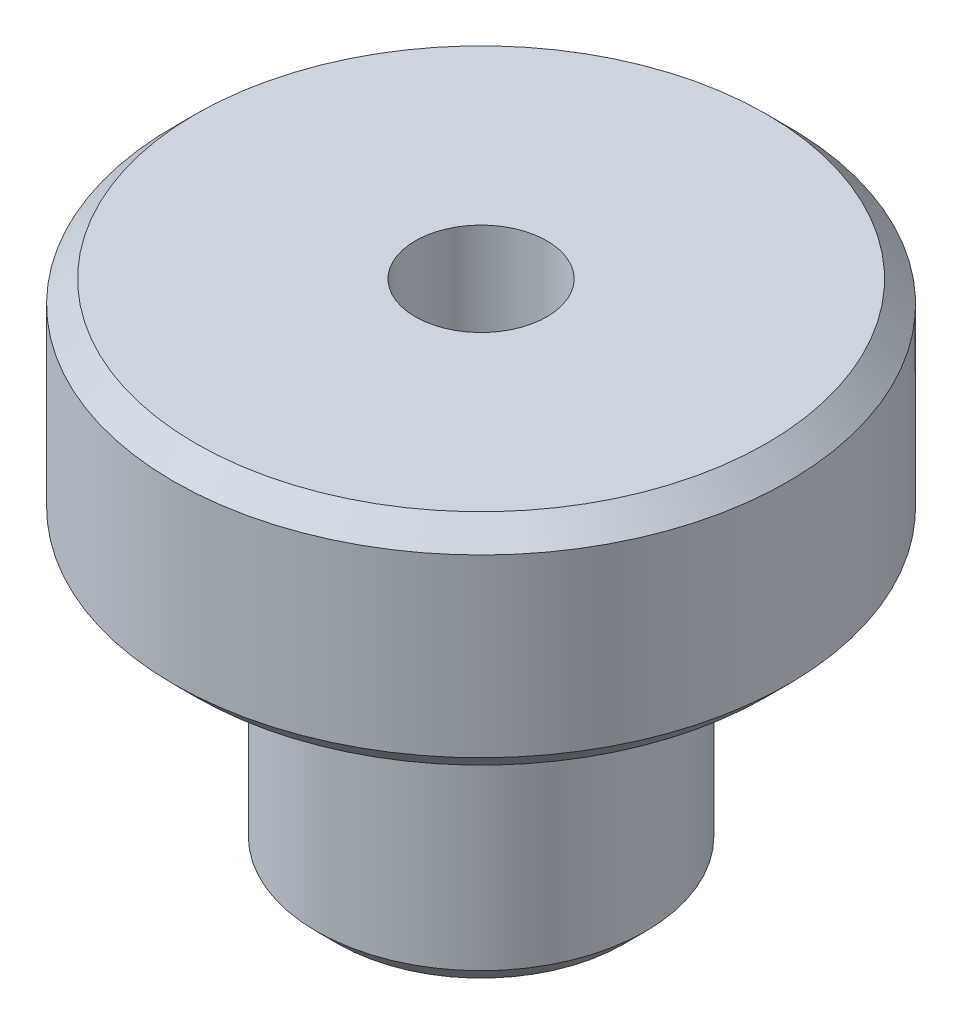
SolidWorks part; units mm, degrees
material "S45C"
ref_plane "Front Plane" through (0, 0, 0) normal (0, 0, 1) x (1, 0, 0)
ref_plane "Top Plane" through (0, 0, 0) normal (0, 1, 0) x (1, 0, 0)
ref_plane "Right Plane" through (0, 0, 0) normal (1, 0, 0) x (0, 0, -1)
sketch "Sketch1" plane through (0, 0, 0) normal (0, 1, 0) x (1, 0, 0)
  circle A0 centre (0, 0) radius 3
  circle A1 centre (0, 0) radius 7.5
  dimension "D1" = 6
  dimension "D2" = 15
extrude "Boss-Extrude1" add sketch "Sketch1" along normal blind 23
sketch "Sketch2" plane through (0, 23, 0) normal (0, 1, 0) x (1, 0, 0)
  circle A0 centre (0, 0) radius 3 construction
  circle A1 centre (0, 0) radius 3
  circle A2 centre (0, 0) radius 14
  dimension "D1" = 28
extrude "Boss-Extrude2" add sketch "Sketch2" against normal blind 10
chamfer "Chamfer1" distance 1 angle 45 3 edges at (0, 13, 14) (0, 23, 14) (0, 0, 7.5)
sketch "Sketch3" plane through (0, 0, 0) normal (1, 0, 0) x (0, 0, -1)
  circle A0 centre (0, 7.0396) radius 2
  dimension "D1" = 4
extrude "Cut-Extrude1" cut sketch "Sketch3" against normal blind 15
